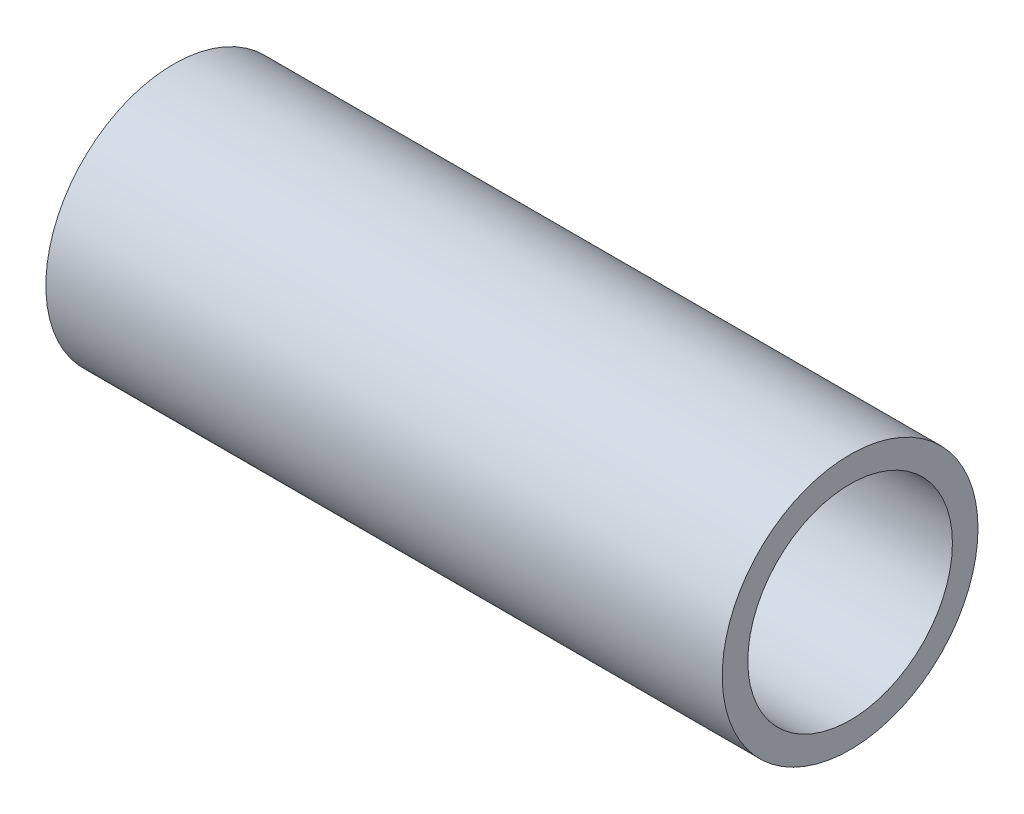
SolidWorks part; units mm, degrees
ref_plane "前视基准面" through (0, 0, 0) normal (0, 0, 1) x (1, 0, 0)
ref_plane "上视基准面" through (0, 0, 0) normal (0, 1, 0) x (1, 0, 0)
ref_plane "右视基准面" through (0, 0, 0) normal (1, 0, 0) x (0, 0, -1)
sketch "草图1" plane through (0, 0, 0) normal (1, 0, 0) x (0, 0, -1)
  circle A0 centre (0, 0) radius 22.5
  circle A1 centre (0, 0) radius 18
extrude "凸台-拉伸1" add sketch "草图1" along normal blind 119
